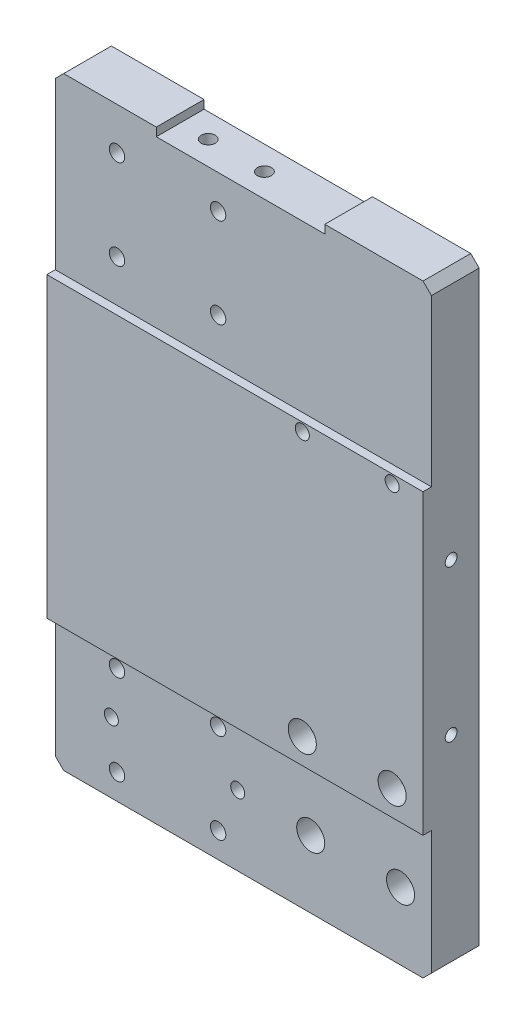
from build123d import *

# Parameters (mm, degrees)
BOSS_EXTRUDE1_DEPTH   = 134
SKETCH2_W             = 60
SKETCH2_H             = 3
CUT_EXTRUDE1_DEPTH    = 134
CHAMFER1_SIZE         = 3
M5_TAPPED_HOLE1_D     = 4.2
M5_TAPPED_HOLE1_DEPTH = 8.7381927
M5_TAPPED_HOLE1_TIP   = 1.2618073
M5_TAPPED_HOLE2_D     = 4.2
M5_TAPPED_HOLE2_DEPTH = 8.7381927
M5_TAPPED_HOLE2_TIP   = 1.2618073
M6_TAPPED_HOLE1_D     = 5
M6_TAPPED_HOLE1_DEPTH = 10.497848452
M6_TAPPED_HOLE1_TIP   = 1.502151548
M6_TAPPED_HOLE2_D     = 5
HOLE1_D               = 5.5
HOLE1_CBORE_D         = 10
HOLE1_CBORE_DEPTH     = 7
CUT_EXTRUDE2_DEPTH    = 3
HOLE2_D               = 5.5
HOLE2_CBORE_D         = 10
HOLE2_CBORE_DEPTH     = 7
HOLE3_D               = 5.5
HOLE3_CBORE_D         = 10
HOLE3_CBORE_DEPTH     = 7
M6_TAPPED_HOLE3_D     = 5


with BuildPart() as part:
    # Sketch1 → Boss-Extrude1 (new body)
    with BuildSketch(Plane(origin=(0, 3.607618474, 0), x_dir=(0, 0, -1), z_dir=(1, 0, 0))):
        Polygon((-22.931720467, -128.880681818), (-22.931720467, -175.880681818), (-5.931720467, -175.880681818), (-5.931720467, 39.119318182), (-22.931720467, 39.119318182), (-22.931720467, -22.880681818), (-25.931720467, -22.880681818), (-25.931720467, -128.880681818), align=None)
    extrude(amount=BOSS_EXTRUDE1_DEPTH)

    # Sketch2 → Cut-Extrude1 (cut)
    with BuildSketch(Plane(origin=(0, 3.607618474, 22.931720467), x_dir=(1, 0, 0), z_dir=(0, 0, 1))):
        with Locations((66, 37.619318182)):
            Rectangle(SKETCH2_W, SKETCH2_H)
    extrude(amount=-CUT_EXTRUDE1_DEPTH, mode=Mode.SUBTRACT)

    # Chamfer1
    chamfer1_edges = [part.edges().sort_by_distance(p)[0] for p in [
        (134, -172.273063344, 14.431720467),
        (134, 42.726936656, 14.431720467),
        (0, 42.726936656, 14.431720467),
        (0, -172.273063344, 14.431720467),
    ]]
    chamfer(chamfer1_edges, length=CHAMFER1_SIZE)

    # M5 Tapped Hole1
    with Locations(Plane(origin=(134, 0, 0), x_dir=(0, 0, -1), z_dir=(1, 0, 0))):
        with Locations((-15.931720467, -45.273063344), (-15.931720467, -99.273063344)):
            Hole(M5_TAPPED_HOLE1_D / 2, depth=M5_TAPPED_HOLE1_DEPTH)
            with Locations((0, 0, -(M5_TAPPED_HOLE1_DEPTH + M5_TAPPED_HOLE1_TIP / 2))):  # 118° drill point
                Cone(0, M5_TAPPED_HOLE1_D / 2, M5_TAPPED_HOLE1_TIP, mode=Mode.SUBTRACT)

    # M5 Tapped Hole2
    with Locations(Plane.ZY):
        with Locations((15.931720467, -45.273063344), (15.931720467, -99.273063344)):
            Hole(M5_TAPPED_HOLE2_D / 2, depth=M5_TAPPED_HOLE2_DEPTH)
            with Locations((0, 0, -(M5_TAPPED_HOLE2_DEPTH + M5_TAPPED_HOLE2_TIP / 2))):  # 118° drill point
                Cone(0, M5_TAPPED_HOLE2_D / 2, M5_TAPPED_HOLE2_TIP, mode=Mode.SUBTRACT)

    # M6 Tapped Hole1
    with Locations(Plane(origin=(0, 39.726936656, 0), x_dir=(1, 0, 0), z_dir=(0, 1, 0))):
        with Locations((66, -14.431720467), (46, -14.431720467)):
            Hole(M6_TAPPED_HOLE1_D / 2, depth=M6_TAPPED_HOLE1_DEPTH)
            with Locations((0, 0, -(M6_TAPPED_HOLE1_DEPTH + M6_TAPPED_HOLE1_TIP / 2))):  # 118° drill point
                Cone(0, M6_TAPPED_HOLE1_D / 2, M6_TAPPED_HOLE1_TIP, mode=Mode.SUBTRACT)

    # M6 Tapped Hole2 (through all)
    with Locations(Plane(origin=(0, 0, 5.931720467), x_dir=(-1, 0, 0), z_dir=(0, 0, -1))):
        with Locations((-123, -22.273063344), (-91, -22.273063344)):
            Hole(M6_TAPPED_HOLE2_D / 2)

    # Hole1 (through all)
    with Locations(Plane(origin=(0, 0, 5.931720467), x_dir=(-1, 0, 0), z_dir=(0, 0, -1))):
        with Locations((-58, 27.726936656), (-22, 27.726936656), (-22, -4.273063344), (-58, -4.273063344), (-58, -131.273063344), (-58, -163.273063344), (-22, -163.273063344), (-22, -131.273063344)):
            CounterBoreHole(HOLE1_D / 2, HOLE1_CBORE_D / 2, HOLE1_CBORE_DEPTH)

    # Sketch17 → Cut-Extrude2 (cut)
    with BuildSketch(Plane(origin=(0, 0, 5.931720467), x_dir=(-1, 0, 0), z_dir=(0, 0, -1))):
        with BuildLine():
            Line((-129, -172.273063344), (-83, -172.273063344))
            Line((-83, -172.273063344), (-83, -77.273063344))
            ThreePointArc((-83, -77.273063344), (-84.464466094, -73.737529438), (-88, -72.273063344))
            Line((-88, -72.273063344), (-124, -72.273063344))
            ThreePointArc((-124, -72.273063344), (-127.535533906, -73.737529438), (-129, -77.273063344))
            Line((-129, -77.273063344), (-129, -172.273063344))
        make_face()
    extrude(amount=-CUT_EXTRUDE2_DEPTH, mode=Mode.SUBTRACT)

    # Hole2 (through all)
    with Locations(Plane.XY.offset(25.931720467)):
        with Locations((91, -116.273063344), (123, -116.273063344)):
            CounterBoreHole(HOLE2_D / 2, HOLE2_CBORE_D / 2, HOLE2_CBORE_DEPTH)

    # Hole3 (through all)
    with Locations(Plane.XY.offset(22.931720467)):
        with Locations((91, -148.273063344), (123, -148.273063344)):
            CounterBoreHole(HOLE3_D / 2, HOLE3_CBORE_D / 2, HOLE3_CBORE_DEPTH)

    # M6 Tapped Hole3 (through all)
    with Locations(Plane.XY.offset(22.931720467)):
        with Locations((20, -147.273063344), (65, -147.273063344)):
            Hole(M6_TAPPED_HOLE3_D / 2)


solid = part.part
